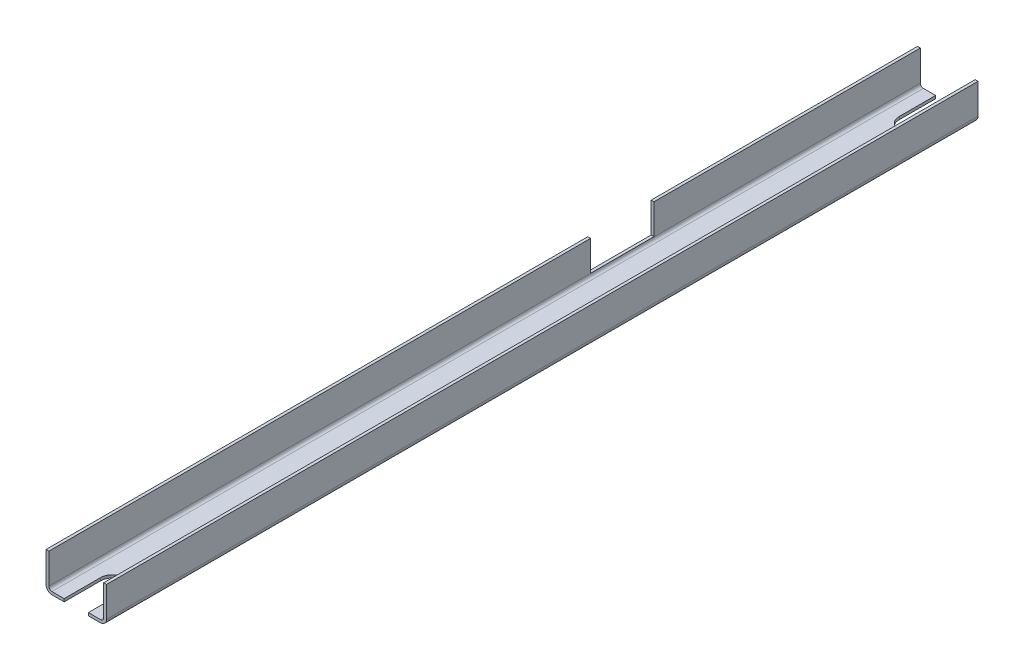
from build123d import *

# Parameters (mm, degrees)
BOSS_EXTRUDE1_DEPTH = 457.2
CUT_EXTRUDE1_REACH  = 460.697
SKETCH2_W           = 33.274
SKETCH2_H           = 15.85
CUT_EXTRUDE2_DEPTH  = 459.696855232


with BuildPart() as part:
    # Sketch1 → Boss-Extrude1 (new body)
    with BuildSketch(Plane.XY):
        with BuildLine():
            Line((30.25, 3.1), (30.25, 19.05))
            Line((30.25, 19.05), (31.75, 19.05))
            Line((31.75, 19.05), (31.75, 3.2))
            ThreePointArc((31.75, 3.2), (30.8127417, 0.9372583), (28.55, 0))
            Line((28.55, 0), (3.2, 0))
            ThreePointArc((3.2, 0), (0.9372583, 0.9372583), (0, 3.2))
            Line((0, 3.2), (0, 19.05))
            Line((0, 19.05), (1.5, 19.05))
            Line((1.5, 19.05), (1.5, 3.1))
            ThreePointArc((1.5, 3.1), (1.96862915, 1.96862915), (3.1, 1.5))
            Line((3.1, 1.5), (28.65, 1.5))
            ThreePointArc((28.65, 1.5), (29.78137085, 1.96862915), (30.25, 3.1))
        make_face()
    extrude(amount=BOSS_EXTRUDE1_DEPTH)

    # Sketch2 → Cut-Extrude1 (cut, up to next)
    with BuildSketch(Plane.ZY, mode=Mode.PRIVATE) as cut_extrude1_sk1:
        with Locations((156.337, 11.125)):
            Rectangle(SKETCH2_W, SKETCH2_H)
    cut_extrude1_tool1 = extrude(cut_extrude1_sk1.sketch, amount=-CUT_EXTRUDE1_REACH, mode=Mode.PRIVATE) & part.part
    add(cut_extrude1_tool1.solids().sort_by_distance((0, 11.125, 156.337))[0], mode=Mode.SUBTRACT)

    # Sketch4 → Cut-Extrude2 (cut, through all)
    with BuildSketch(Plane.XZ):
        with BuildLine():
            Line((9.525, 457.2), (9.525, 438.15))
            ThreePointArc((9.525, 438.15), (15.875, 431.8), (22.225, 438.15))
            Line((22.225, 438.15), (22.225, 457.2))
            Line((22.225, 457.2), (9.525, 457.2))
        make_face()
    cut_extrude2 = extrude(amount=-CUT_EXTRUDE2_DEPTH, mode=Mode.SUBTRACT)

    # Mirror1: Cut-Extrude2 across plane
    add(cut_extrude2.mirror(Plane.XY.offset(228.6)), mode=Mode.SUBTRACT)


solid = part.part
